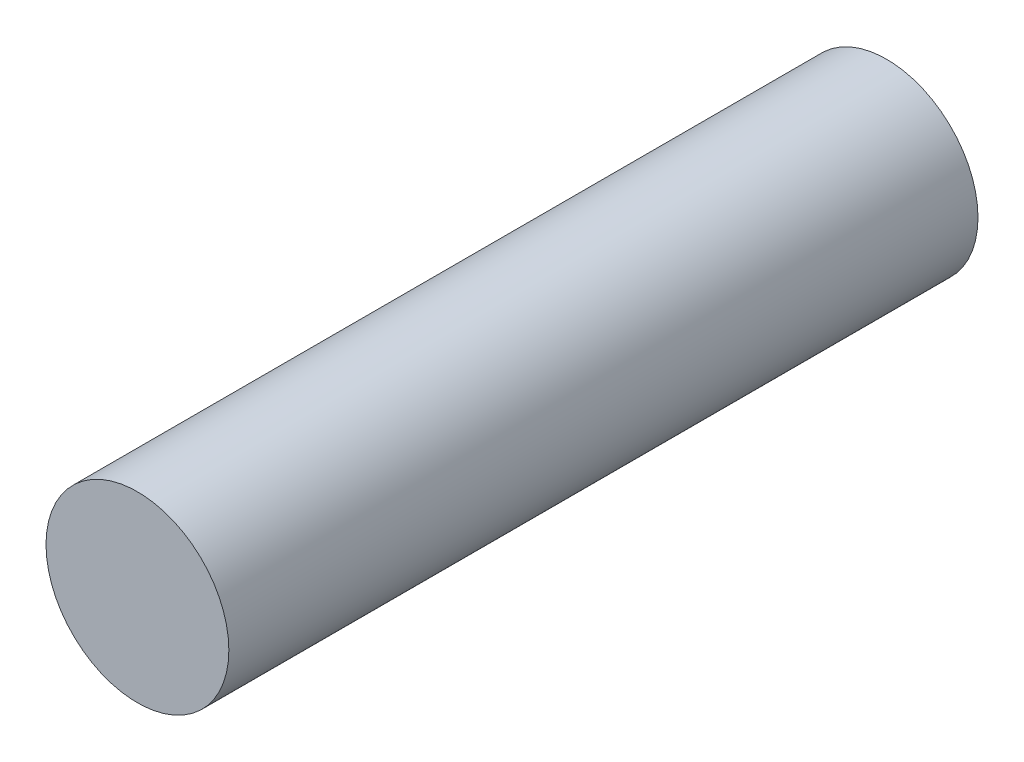
SolidWorks part; units mm, degrees
ref_plane "Front Plane" through (0, 0, 0) normal (0, 0, 1) x (1, 0, 0)
ref_plane "Top Plane" through (0, 0, 0) normal (0, 1, 0) x (1, 0, 0)
ref_plane "Right Plane" through (0, 0, 0) normal (1, 0, 0) x (0, 0, -1)
other "Configuration Table"
sketch "Sketch1" plane through (0, 0, 0) normal (0, 0, 1) x (1, 0, 0)
  circle A1 centre (-27.1889, -16.2883) radius 3.6746
extrude "Boss-Extrude1" add sketch "Sketch1" against normal up to surface (30.1078 mm away)
